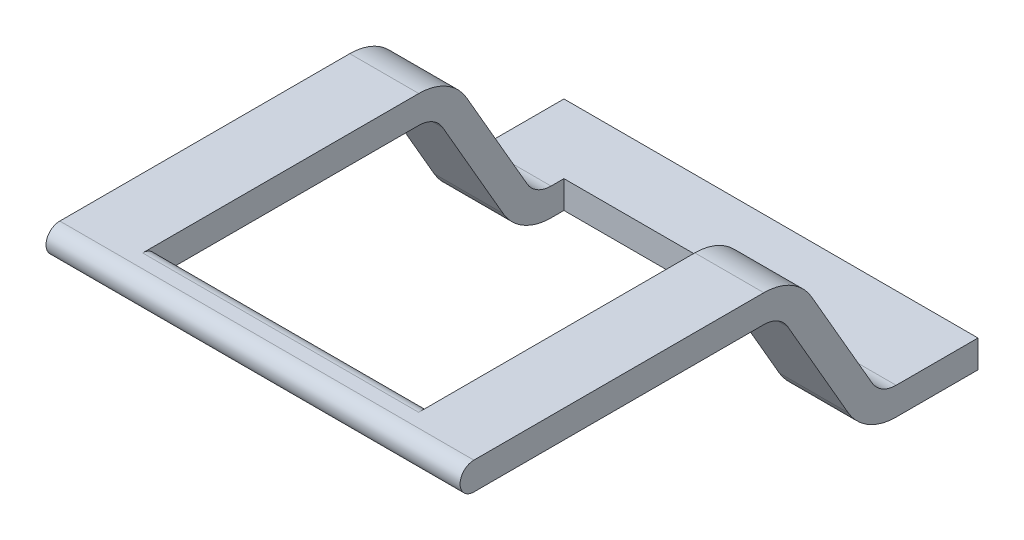
SolidWorks part; units mm, degrees
ref_plane "Front Plane" through (0, 0, 0) normal (0, 0, 1) x (1, 0, 0)
ref_plane "Top Plane" through (0, 0, 0) normal (0, 1, 0) x (1, 0, 0)
ref_plane "Right Plane" through (0, 0, 0) normal (1, 0, 0) x (0, 0, -1)
other "Configuration Table"
ref_plane "Plane1" through (-30, 0, 0) normal (-1, 0, 0) x (0, -1, 0)
sketch "Sketch1" plane through (-30, 0, 0) normal (-1, 0, 0) x (0, -1, 0)
  line L0 (0, -1) -> (0, -2)
  line L1 (2, -2) -> (2, -1)
  arc A0 (0, -2) -> (2, -2) centre (1, -2) ccw
  arc A1 (2, -1) -> (0, -1) centre (1, -1) ccw
extrude "Boss-Extrude1" add sketch "Sketch1" against normal blind 30
sketch "Sketch2" plane through (0, 0, 0) normal (1, 0, 0) x (0, 0, -1)
  line L0 (2, 0) -> (2, -2)
  arc A0 (2, -2) -> (2, 0) centre (2, -1) ccw
extrude "Cut-Extrude1" cut sketch "Sketch2" against normal blind 5
sketch "Sketch3" plane through (0, 0, -2) normal (0, 0, -1) x (-1, 0, 0)
  line L0 (5, -2) -> (0, -2)
  line L1 (0, -2) -> (0, 0)
  line L2 (0, 0) -> (5, 0)
  line L3 (5, 0) -> (5, -1)
  line L4 (5, -1) -> (5, -2)
extrude "Boss-Extrude2" add sketch "Sketch3" along normal blind 1
sketch "Sketch4" plane through (0, 0, -3) normal (0, 0, -1) x (-1, 0, 0)
  line L0 (5, -2) -> (0, -2)
  line L1 (0, -2) -> (0, 0)
  line L2 (0, 0) -> (5, 0)
  line L3 (5, 0) -> (5, -2)
extrude "Boss-Extrude3" add sketch "Sketch4" along normal blind 20.1634
sketch "Sketch5" plane through (0, 0, -23.1634) normal (0, 0, -1) x (-1, 0, 0)
  line L0 (5, 0) -> (5, -10.599)
  line L1 (5, -10.599) -> (0, -10.599)
  line L2 (0, -10.599) -> (0, 0)
  line L3 (0, 0) -> (5, 0)
extrude "Boss-Extrude4" add sketch "Sketch5" along normal blind 1.1547
sketch "Sketch6" plane through (-30, 0, 0) normal (-1, 0, 0) x (0, 0, 1)
  line L0 (-2, -2) -> (-2, 0)
  arc A0 (-2, 0) -> (-2, -2) centre (-2, -1) ccw
extrude "Cut-Extrude2" cut sketch "Sketch6" against normal blind 5
sketch "Sketch7" plane through (0, 0, -2) normal (0, 0, -1) x (-1, 0, 0)
  line L0 (30, -2) -> (25, -2)
  line L1 (25, -2) -> (25, -1)
  line L2 (25, -1) -> (25, 0)
  line L3 (25, 0) -> (30, 0)
  line L4 (30, 0) -> (30, -2)
extrude "Boss-Extrude5" add sketch "Sketch7" along normal blind 1
sketch "Sketch8" plane through (0, 0, -3) normal (0, 0, -1) x (-1, 0, 0)
  line L0 (30, -2) -> (25, -2)
  line L1 (25, -2) -> (25, 0)
  line L2 (25, 0) -> (30, 0)
  line L3 (30, 0) -> (30, -2)
extrude "Boss-Extrude6" add sketch "Sketch8" along normal blind 20.1634
sketch "Sketch9" plane through (0, 0, -23.1634) normal (0, 0, -1) x (-1, 0, 0)
  line L0 (30, 0) -> (30, -10.599)
  line L1 (30, -10.599) -> (25, -10.599)
  line L2 (25, -10.599) -> (25, 0)
  line L3 (25, 0) -> (30, 0)
extrude "Boss-Extrude7" add sketch "Sketch9" along normal blind 1.1547
sketch "Sketch10" plane through (0, -10.599, 0) normal (0, -1, 0) x (1, 0, 0)
  line L0 (0, -23.1634) -> (0, -37.5257)
  line L1 (0, -37.5257) -> (-30, -37.5257)
  line L2 (-30, -37.5257) -> (-30, -23.1634)
  line L3 (-30, -23.1634) -> (-25, -23.1634)
  line L4 (-25, -23.1634) -> (-25, -32.5257)
  line L5 (-25, -32.5257) -> (-5, -32.5257)
  line L6 (-5, -32.5257) -> (-5, -23.1634)
  line L7 (-5, -23.1634) -> (0, -23.1634)
extrude "Boss-Extrude8" add sketch "Sketch10" along normal blind 2
draft "Draft1" type of draft neutral plane draft angle 30 faces to draft 2 face at (-2.5, -5.2995, -24.3181) face at (-27.5, -5.2995, -24.3181) neutral plane through (0, 0, -1) neutral plane normal (0, 1, 0) parameters "D1"=30
draft "Draft2" type of draft neutral plane draft angle 30 faces to draft 2 face at (-27.5, -7.2995, -23.1634) face at (-2.5, -7.2995, -23.1634) neutral plane through (0, -2, -2) neutral plane normal (0, -1, 0) parameters "D1"=30
fillet "Fillet1" radius 2 4 edges at (-27.5, -2, -23.1634) (-2.5, -2, -23.1634) (-27.5, -10.599, -30.4374) (-2.5, -10.599, -30.4374)
fillet "Fillet2" radius 4 4 edges at (-27.5, 0, -24.3181) (-2.5, 0, -24.3181) (-2.5, -12.599, -29.2827) (-27.5, -12.599, -29.2827)
